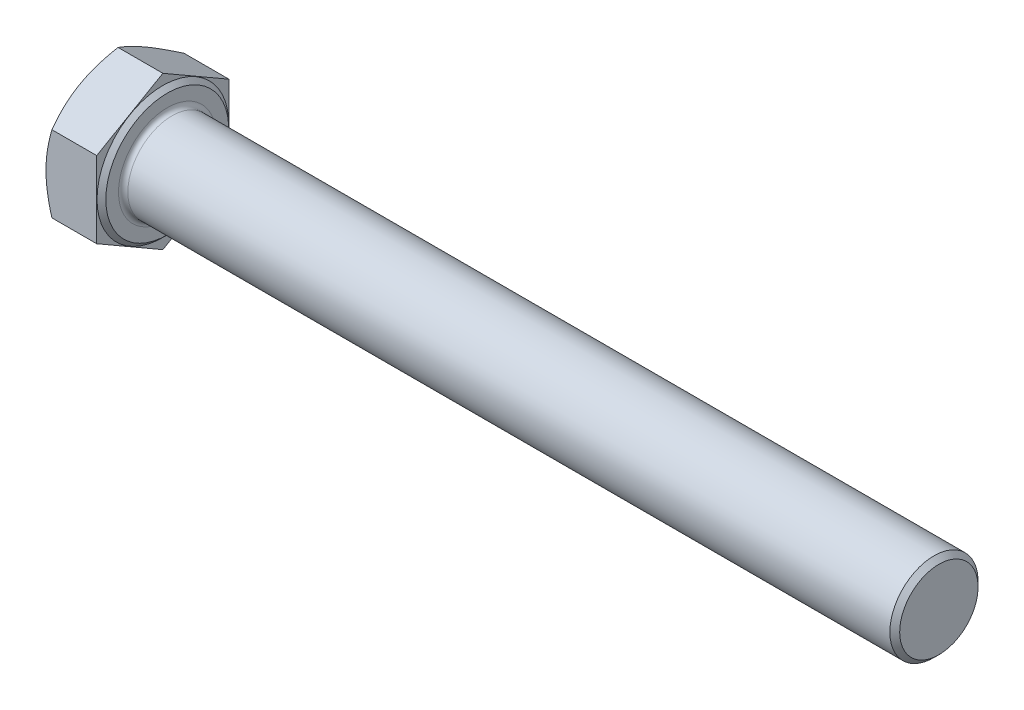
from build123d import *

# Parameters (mm, degrees)
BOSS_EXTRUDE1_DEPTH = 10
SKETCH4_R           = 26.75
SKETCH4_R_2         = 12
CUT_EXTRUDE1_DEPTH  = 1.25
CUT_EXTRUDE1_DRAFT  = -60
CHAMFER2_SIZE       = 0.888888889


with BuildPart() as part:
    # Sketch3 → Boss-Extrude1 (new body)
    with BuildSketch(Plane(origin=(0, 0, 0), x_dir=(0, 0, -1), z_dir=(1, 0, 0))):
        Polygon((12, 6.92820323), (0, 13.856406461), (-12, 6.92820323), (-12, -6.92820323), (0, -13.856406461), (12, -6.92820323), align=None)
    extrude(amount=BOSS_EXTRUDE1_DEPTH)


with BuildPart() as cut_extrude1_tool:
    # Sketch4 → Cut-Extrude1 (with draft: the straight prism first)
    with BuildSketch(Plane.ZY):
        Circle(SKETCH4_R)
        Circle(SKETCH4_R_2, mode=Mode.SUBTRACT)
    extrude(amount=-CUT_EXTRUDE1_DEPTH)
    # Cut-Extrude1: the draft: its side faces are tilted about the plane it starts from
    cut_extrude1_sides = [cut_extrude1_tool.faces().sort_by_distance(p)[0] for p in [
        (0.625, 0, -26.75),
        (0.625, 0, -12),
    ]]
    draft(cut_extrude1_sides, Plane.ZY, CUT_EXTRUDE1_DRAFT)


with BuildPart() as part_1:
    add(part.part)

    # Cut-Extrude1: cut by cut_extrude1_tool
    add(cut_extrude1_tool.part, mode=Mode.SUBTRACT)

    # Sketch5 → Revolve1 (revolve)
    with BuildSketch(Plane.XY, mode=Mode.PRIVATE) as revolve1_sk:
        with BuildLine():
            Line((10.85, 8), (150, 8))
            Line((150, 8), (150, 0))
            Line((150, 0), (10, 0))
            Line((10, 0), (10, 8.85))
            ThreePointArc((10, 8.85), (10.248959236, 8.248959236), (10.85, 8))
        make_face()
    revolve(revolve1_sk.sketch.rotate(Axis((10, 0, 0), (1, 0, 0)), 90), axis=Axis((10, 0, 0), (1, 0, 0)))

    # Chamfer2
    chamfer2_edges = [part_1.edges().sort_by_distance(p)[0] for p in [
        (150, 0, -8),
    ]]
    chamfer(chamfer2_edges, length=CHAMFER2_SIZE)

    # Sketch7 → Cut-Revolve1 (revolve, cut)
    with BuildSketch(Plane.XY, mode=Mode.PRIVATE) as cut_revolve1_sk:
        Polygon((10, 11.145), (9.2, 11.945), (9.2, 26.75), (10, 26.75), align=None)
    revolve(cut_revolve1_sk.sketch.rotate(Axis((0, 0, 0), (1, 0, 0)), 90), axis=Axis((0, 0, 0), (1, 0, 0)), mode=Mode.SUBTRACT)


solid = part_1.part
